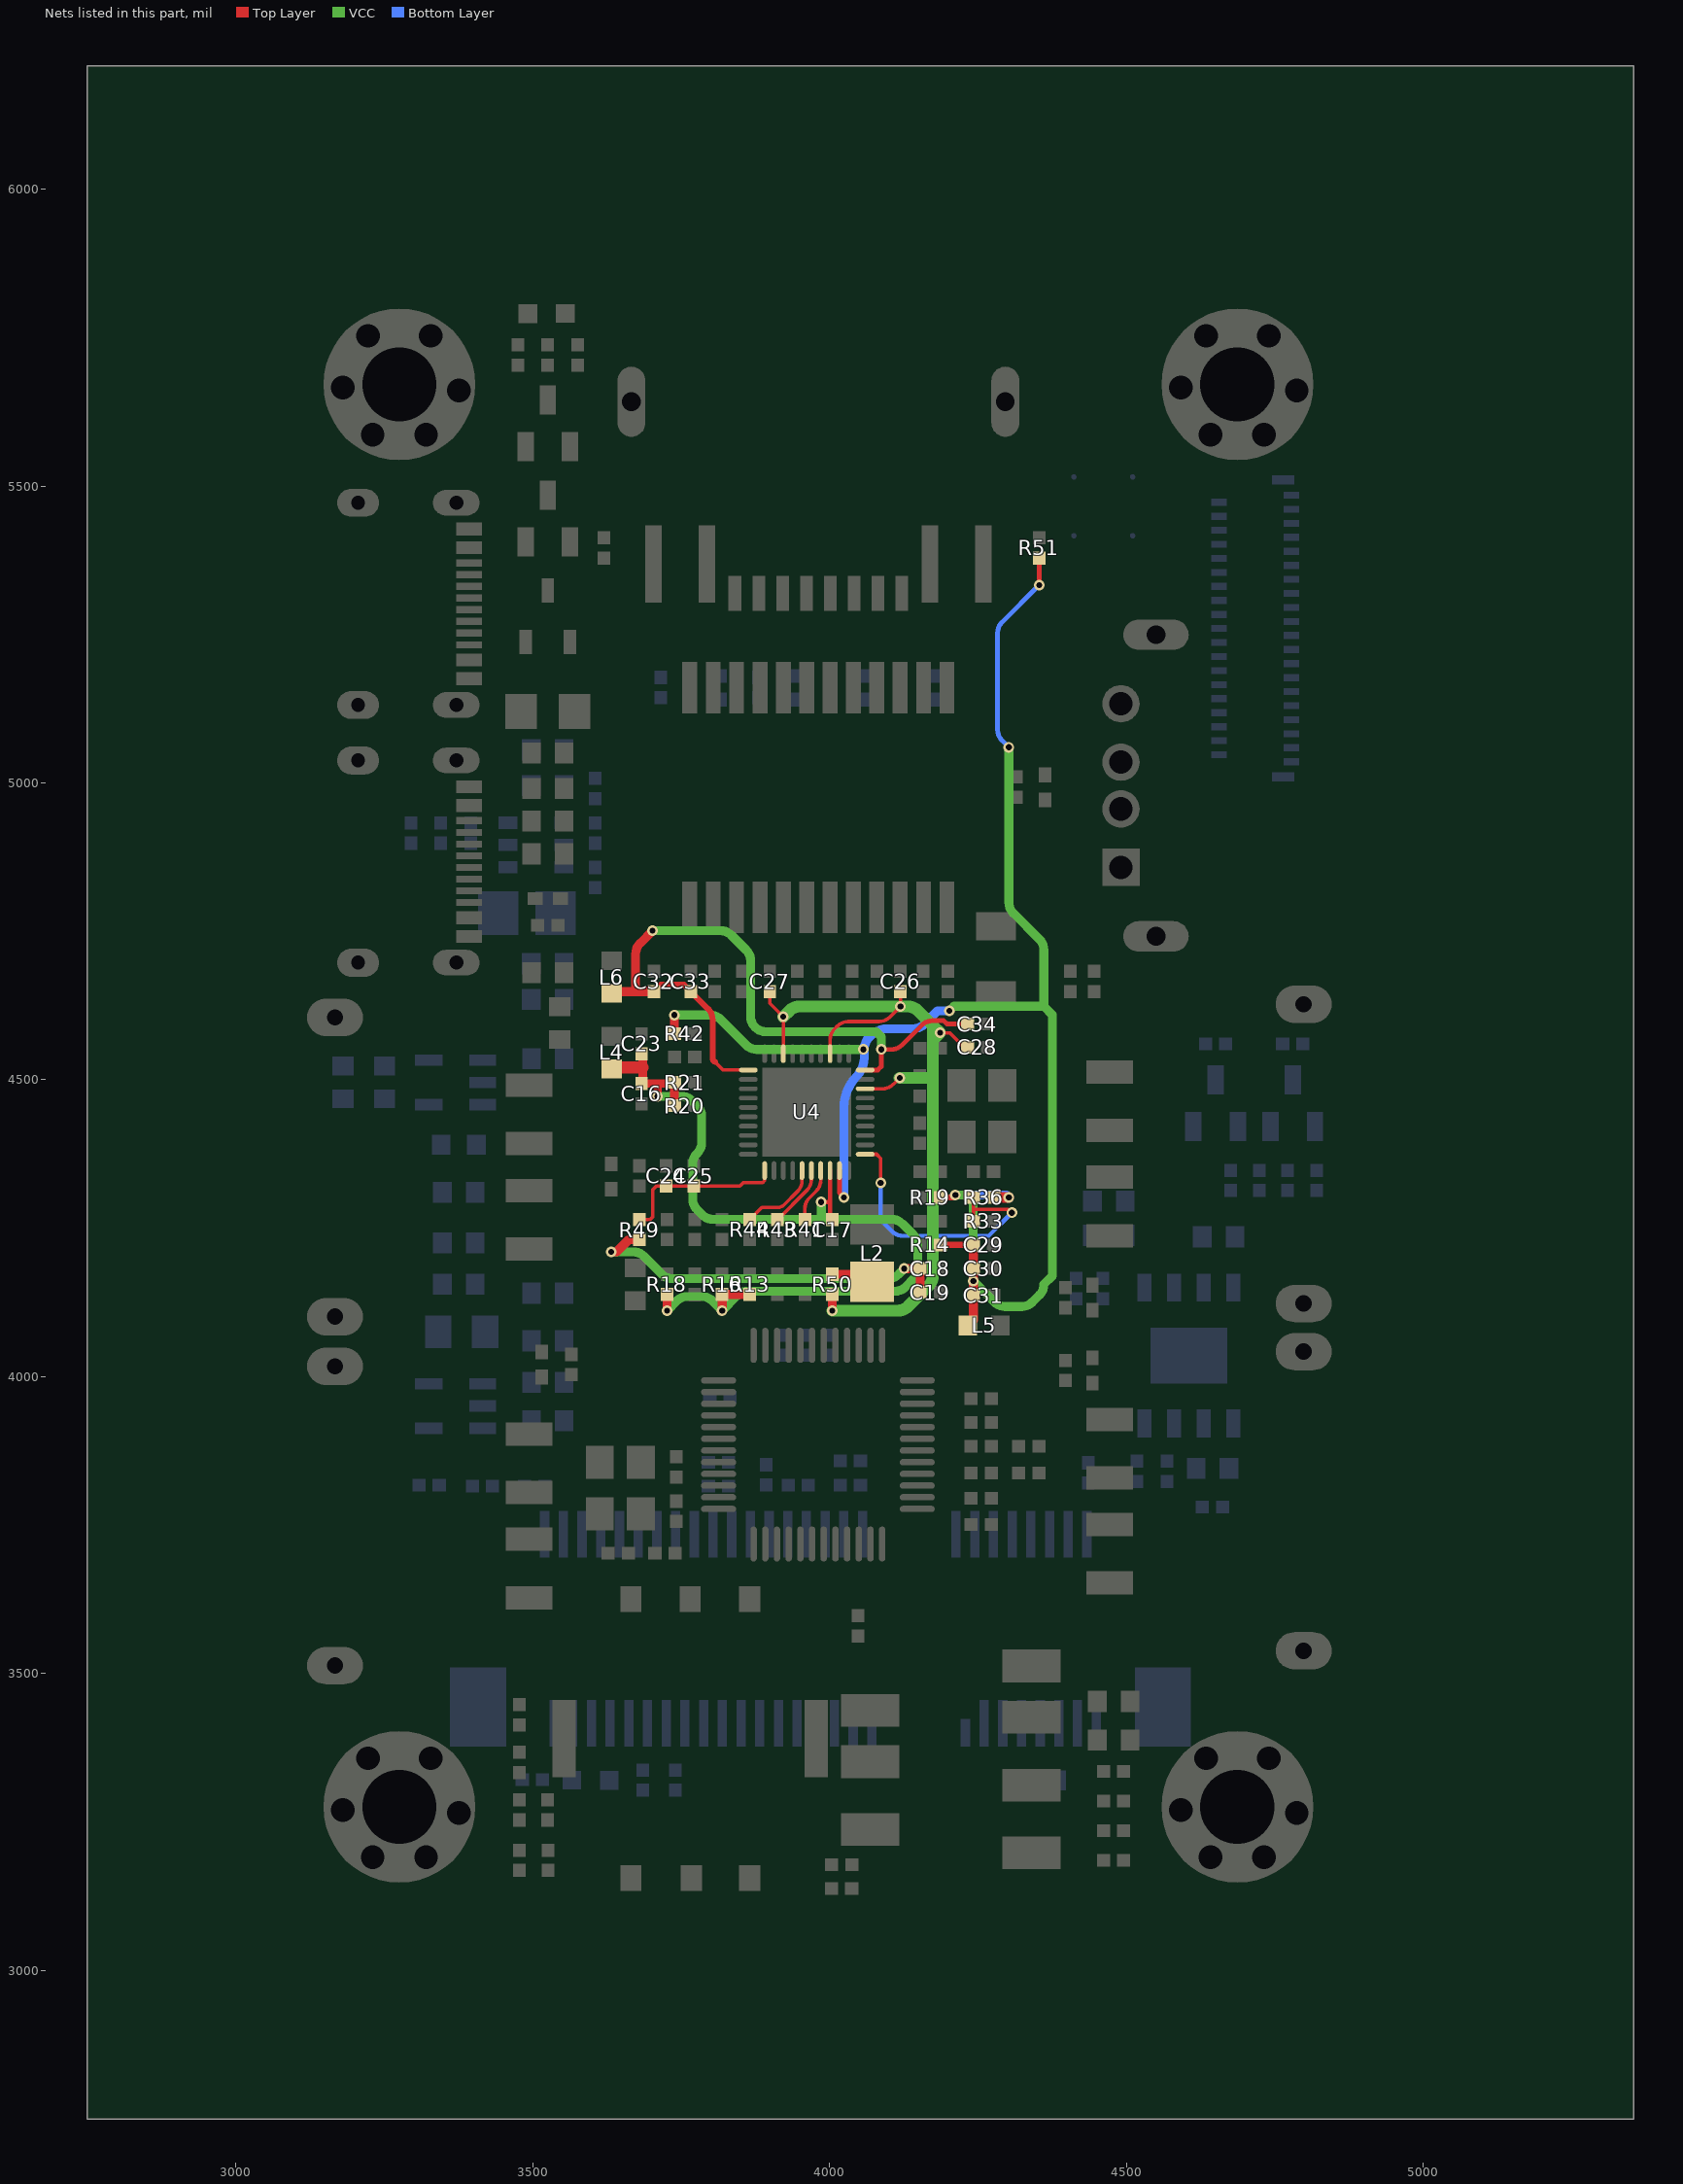
[diagram p0: the nets of this part, all layers, seen from the top]
# Altium PCB MISC84334.PcbDoc (part 3 of 8)
Units mil, origin at the board's own origin, x right, y up, seen from the top; angles counter-clockwise.
Board outline 2605.13 x 3457.4 mil, 4 copper layers (Top Layer, GND, VCC, Bottom Layer), stack 62.447 mil thick; 209 components, 149 nets, 735 pads, 529 vias.

## Footprints (in the part's own frame and the unit in brackets; to place one, negate y for a bottom-side part, rotate by r counter-clockwise, add the part's x,y. Pads: shape width x height; smd on the part's side, far side on the other; paste and mask are expansions set on the pad) (continued)
PCI-SMD_1775862-2 [mm]
  rect 0.4x2 smd: 1(11.8,4.05) 2(11.4,-4.05) 3(11,4.05) 4(10.6,-4.05) 5(10.2,4.05) 6(9.8,-4.05) 7(9.4,4.05) 8(9,-4.05) 9(8.6,4.05) 10(8.2,-4.05) 11(7.8,4.05) 12(7.4,-4.05) 13(7,4.05) 14(6.6,-4.05) 16(5.8,-4.05) 17(2.2,4.05) 18(1.8,-4.05) 19(1.4,4.05) 20(1,-4.05) 21(0.6,4.05) 22(0.2,-4.05) 23(-0.2,4.05) 24(-0.6,-4.05) 25(-1,4.05) 26(-1.4,-4.05) 27(-1.8,4.05) 28(-2.2,-4.05) 29(-2.6,4.05) 30(-3,-4.05) 31(-3.4,4.05) 32(-3.8,-4.05) 33(-4.2,4.05) 34(-4.6,-4.05) 35(-5,4.05) 36(-5.4,-4.05) 37(-5.8,4.05) 38(-6.2,-4.05) 39(-6.6,4.05) 40(-7,-4.05) 41(-7.4,4.05) 42(-7.8,-4.05) 43(-8.2,4.05) 44(-8.6,-4.05) 45(-9,4.05) 46(-9.4,-4.05) 47(-9.8,4.05) 48(-10.2,-4.05) 49(-10.6,4.05) 50(-11,-4.05) 51(-11.4,4.05) 52(-11.8,-4.05)
  rect 0.4x1.2 smd: 15(6.2,4.45)
  rect 2.4x3.4 smd: 53(-14.65,3.35) 53(14.65,3.35)
  Board Outline Layer circle w0.003: c-12.5,0.05 r0.6
  Board Outline Layer circle w0.003: c12.5,0.05 r0.9
  Board Outline Layer region: -11.9,0.05 -11.96,0.31 -12.126,0.519 -12.367,0.635 -12.634,0.635 -12.874,0.519 -13.041,0.31 -13.1,0.05 -13.1,0.05 -13.041,-0.21 -12.874,-0.419 -12.634,-0.535 -12.367,-0.535 -12.126,-0.419 -11.96,-0.21 -11.9,0.05
  Board Outline Layer region: -11.9,0.05 -11.909,0.154 -11.936,0.255 -11.98,0.35 -12.04,0.436 -12.114,0.51 -12.2,0.57 -12.295,0.614 -12.396,0.641 -12.5,0.65 -12.604,0.641 -12.705,0.614 -12.8,0.57 -12.886,0.51 -12.96,0.436 -13.02,0.35 -13.064,0.255 -13.091,0.154 -13.1,0.05 -13.091,-0.054 -13.064,-0.155 -13.02,-0.25 -12.96,-0.336 -12.886,-0.41 -12.8,-0.47 -12.705,-0.514 -12.604,-0.541 -12.5,-0.55 -12.396,-0.541 -12.295,-0.514 -12.2,-0.47 -12.114,-0.41 -12.04,-0.336 -11.98,-0.25 -11.936,-0.155 -11.909,-0.054
  Board Outline Layer region: 13.4,0.05 13.311,0.441 13.061,0.754 12.7,0.927 12.3,0.927 11.939,0.754 11.689,0.441 11.6,0.05 11.6,0.05 11.689,-0.34 11.939,-0.654 12.3,-0.827 12.7,-0.827 13.061,-0.654 13.311,-0.34 13.4,0.05
  Board Outline Layer region: 13.4,0.05 13.39,0.184 13.36,0.315 13.311,0.441 13.244,0.557 13.16,0.662 13.061,0.754 12.95,0.829 12.829,0.888 12.7,0.927 12.567,0.948 12.433,0.948 12.3,0.927 12.171,0.888 12.05,0.829 11.939,0.754 11.84,0.662 11.756,0.557 11.689,0.441 11.64,0.315 11.61,0.184 11.6,0.05 11.61,-0.084 11.64,-0.215 11.689,-0.34 11.756,-0.457 11.84,-0.562 11.939,-0.654 12.05,-0.729 12.171,-0.788 12.3,-0.827 12.433,-0.847 12.567,-0.847 12.7,-0.827 12.829,-0.788 12.95,-0.729 13.061,-0.654 13.16,-0.562 13.244,-0.457 13.311,-0.34 13.36,-0.215 13.39,-0.084
  Multi-Layer board cut-out: -11.9,0.05 -11.96,0.31 -12.126,0.519 -12.367,0.635 -12.634,0.635 -12.874,0.519 -13.041,0.31 -13.1,0.05 -13.1,0.05 -13.041,-0.21 -12.874,-0.419 -12.634,-0.535 -12.367,-0.535 -12.126,-0.419 -11.96,-0.21 -11.9,0.05
  Multi-Layer board cut-out: 13.4,0.05 13.311,0.441 13.061,0.754 12.7,0.927 12.3,0.927 11.939,0.754 11.689,0.441 11.6,0.05 11.6,0.05 11.689,-0.34 11.939,-0.654 12.3,-0.827 12.7,-0.827 13.061,-0.654 13.311,-0.34 13.4,0.05
  silkscreen extent -15,-4.71 15,4.08
R0402 [mm]
  rect 0.566x0.54 smd paste-100 mask+0.051: 1(-0.433,0) 2(0.433,0)
r0402 [mm]
  rect 0.566x0.54 smd paste-100 mask+0.051: 1(-0.433,0) 2(0.433,0)
r0603#1 [mm]
  rect 0.8x0.9 smd: 1(-0.7,0) 2(0.7,0)
r0603#2 [mm]
  rect 0.8x0.9 smd: 1(-0.698,0) 2(0.702,0)
R0603 [mil]
  rect 31.75x34.02 smd paste-3937.01 mask+2: 1(-29.66,0) 2(29.66,0)
R0805 [mm]
  rect 1.133x1.377 smd paste-100 mask+0.051: 1(-1,0) 2(1,0)
r1206 [mil]
  rect 47.54x66.97 smd paste-3937.01 mask+2: 1(-58.22,0) 2(58.22,0)
RJ45-TH_RC01812 [mm]
  rect 0.55x1.5 smd paste-100 mask+0.05: 1(-3.57,-4.1) 2(-2.55,-4.1) 3(-1.53,-4.1) 4(-0.51,-4.1) 5(0.51,-4.1) 6(1.53,-4.1) 7(2.55,-4.1) 8(3.57,-4.1)
  rect 0.7x3.3 smd paste-100 mask+0.05: 9(-7.06,-2.845) 10(-4.77,-2.845) 11(4.77,-2.845) 12(7.06,-2.845)
  oval 1.2x3 hole 0.8 slot 2.2 at 90 deg paste+0 mask+0.05: 13(-8,4.1) 14(8,4.1)
  Board Outline Layer lines w0.254: -8.128,9.271 -6.985,9.271 -6.985,-0.381 6.985,-0.381 6.985,9.271 8.128,9.271
  silkscreen extent -8.1,-3.14 8.13,12.11
SIM-SMD_SMN-304 [mm]
  rect 1x3.29 smd: 1(-5.39,0) 2(5.39,0)
  rect 0.9x1.1 smd: C1(2.54,-5.975) C2(0.051,-5.975) C3(-2.54,-5.975) C5(2.54,5.975) C6(0,5.975) C7(-2.54,5.975)
  Board Outline Layer circle w0.003: c-4.34,-4.155 r0.5
  Board Outline Layer circle w0.003: c4.66,4.145 r0.4
  Board Outline Layer region: -3.84,-4.155 -3.889,-4.372 -4.028,-4.546 -4.229,-4.643 -4.451,-4.643 -4.652,-4.546 -4.79,-4.372 -4.84,-4.155 -4.84,-4.155 -4.79,-3.938 -4.652,-3.764 -4.451,-3.668 -4.229,-3.668 -4.028,-3.764 -3.889,-3.938 -3.84,-4.155
  Board Outline Layer region: -3.84,-4.155 -3.85,-4.253 -3.878,-4.346 -3.924,-4.433 -3.986,-4.509 -4.062,-4.571 -4.149,-4.617 -4.242,-4.645 -4.34,-4.655 -4.438,-4.645 -4.531,-4.617 -4.618,-4.571 -4.694,-4.509 -4.756,-4.433 -4.802,-4.346 -4.83,-4.253 -4.84,-4.155 -4.83,-4.058 -4.802,-3.964 -4.756,-3.877 -4.694,-3.802 -4.618,-3.739 -4.531,-3.693 -4.438,-3.665 -4.34,-3.655 -4.242,-3.665 -4.149,-3.693 -4.062,-3.739 -3.986,-3.802 -3.924,-3.877 -3.878,-3.964 -3.85,-4.058
  Board Outline Layer region: 5.06,4.145 5.02,3.972 4.909,3.832 4.749,3.755 4.571,3.755 4.411,3.832 4.3,3.972 4.26,4.145 4.26,4.145 4.3,4.319 4.411,4.458 4.571,4.535 4.749,4.535 4.909,4.458 5.02,4.319 5.06,4.145
  Board Outline Layer region: 5.06,4.145 5.05,4.056 5.02,3.972 4.973,3.896 4.909,3.832 4.834,3.785 4.749,3.755 4.66,3.745 4.571,3.755 4.486,3.785 4.411,3.832 4.347,3.896 4.3,3.972 4.27,4.056 4.26,4.145 4.27,4.234 4.3,4.319 4.347,4.395 4.411,4.458 4.486,4.506 4.571,4.535 4.66,4.545 4.749,4.535 4.834,4.506 4.909,4.458 4.973,4.395 5.02,4.319 5.05,4.234
  Multi-Layer board cut-out: -3.84,-4.155 -3.889,-4.372 -4.028,-4.546 -4.229,-4.643 -4.451,-4.643 -4.652,-4.546 -4.79,-4.372 -4.84,-4.155 -4.84,-4.155 -4.79,-3.938 -4.652,-3.764 -4.451,-3.668 -4.229,-3.668 -4.028,-3.764 -3.889,-3.938 -3.84,-4.155
  Multi-Layer board cut-out: 5.06,4.145 5.02,3.972 4.909,3.832 4.749,3.755 4.571,3.755 4.411,3.832 4.3,3.972 4.26,4.145 4.26,4.145 4.3,4.319 4.411,4.458 4.571,4.535 4.749,4.535 4.909,4.458 5.02,4.319 5.06,4.145
  silkscreen extent -5.03,-6.15 5.11,6.16
SMD-24_L15.1-W7.1-P1.00-LS10.0-BL [mm]
  rect 0.64x2.2 smd: 1(-5.5,-4.7) 2(-4.5,-4.7) 3(-3.5,-4.7) 4(-2.5,-4.7) 5(-1.5,-4.7) 6(-0.5,-4.7) 7(0.5,-4.7) 8(1.5,-4.7) 9(2.5,-4.7) 10(3.5,-4.7) 11(4.5,-4.7) 12(5.5,-4.7) 13(5.5,4.7) 14(4.5,4.7) 15(3.5,4.7) 16(2.5,4.7) 17(1.5,4.7) 18(0.5,4.7) 19(-0.5,4.7) 20(-1.5,4.7) 21(-2.5,4.7) 22(-3.5,4.7) 23(-4.5,4.7) 24(-5.5,4.7)
  silkscreen extent -7.6,-5 7.6,3.6
SMD_BD4.4-L4.4-D2.8 [mil]
  round 9.02 smd: 1(-49.52,49.5) 1(-49.51,-49.52) 1(49.5,49.52) 1(49.52,-49.5)
  Top Layer region: 3.8,90.43 3.8,60.9 6.05,60.72 8.3,60.45 10.53,60.1 12.75,59.67 14.95,59.15 17.13,58.56 19.29,57.88 21.43,57.13 23.53,56.29 25.6,55.38 27.63,54.39 29.63,53.33 31.59,52.2 33.5,50.99 35.36,49.71 37.18,48.37 38.95,46.96 40.66,45.48 42.32,43.94 43.92,42.34 45.46,40.68 46.94,38.97 48.35,37.2 49.69,35.39 50.97,33.52 52.18,31.61 53.31,29.65 54.37,27.65 55.36,25.62 56.27,23.55 57.11,21.45 57.86,19.31 58.54,17.15 59.13,14.97 59.65,12.77 60.08,10.55 60.43,8.32 60.7,6.07 60.88,3.82 90.41,3.82 90.25,6.56 90.01,9.29 89.69,12.02 89.28,14.73 88.79,17.43 88.22,20.12 87.57,22.79 86.84,25.43 86.02,28.05 85.13,30.65 84.16,33.22 83.12,35.76 81.99,38.26 80.79,40.73 79.52,43.16 78.17,45.56 76.76,47.91 75.27,50.21 73.71,52.47 72.08,54.69 70.39,56.85 68.63,58.96 66.81,61.01 64.93,63.01 62.99,64.95 60.99,66.84 58.94,68.65 56.83,70.41 54.67,72.1 52.45,73.73 50.19,75.29 47.89,76.78 45.54,78.19 43.14,79.54 40.71,80.81 38.24,82.01 35.74,83.14 33.2,84.18 30.63,85.15 28.03,86.04 25.41,86.86 22.77,87.59 20.1,88.24 17.41,88.81 14.71,89.3 12,89.71 9.27,90.03 6.54,90.27
  Top Layer region: -3.8,-90.43 -3.8,-60.9 -6.06,-60.72 -8.3,-60.45 -10.54,-60.1 -12.76,-59.67 -14.96,-59.15 -17.14,-58.56 -19.3,-57.88 -21.43,-57.13 -23.53,-56.29 -25.6,-55.38 -27.64,-54.4 -29.64,-53.33 -31.59,-52.2 -33.51,-50.99 -35.37,-49.71 -37.19,-48.37 -38.96,-46.96 -40.67,-45.48 -42.33,-43.94 -43.93,-42.34 -45.47,-40.68 -46.94,-38.97 -48.35,-37.2 -49.7,-35.39 -50.98,-33.52 -52.18,-31.61 -53.32,-29.65 -54.38,-27.65 -55.37,-25.62 -56.28,-23.55 -57.11,-21.45 -57.87,-19.31 -58.55,-17.15 -59.14,-14.97 -59.66,-12.77 -60.09,-10.55 -60.44,-8.32 -60.7,-6.07 -60.89,-3.82 -90.42,-3.82 -90.26,-6.56 -90.02,-9.29 -89.69,-12.02 -89.28,-14.73 -88.8,-17.43 -88.23,-20.12 -87.57,-22.79 -86.84,-25.43 -86.03,-28.05 -85.14,-30.65 -84.17,-33.22 -83.12,-35.76 -82,-38.26 -80.8,-40.73 -79.53,-43.16 -78.18,-45.56 -76.76,-47.91 -75.27,-50.21 -73.72,-52.47 -72.09,-54.69 -70.4,-56.85 -68.64,-58.96 -66.82,-61.01 -64.94,-63.01 -63,-64.95 -61,-66.84 -58.94,-68.65 -56.83,-70.41 -54.67,-72.1 -52.46,-73.73 -50.2,-75.29 -47.89,-76.78 -45.54,-78.19 -43.15,-79.54 -40.72,-80.81 -38.25,-82.01 -35.74,-83.14 -33.2,-84.18 -30.64,-85.15 -28.04,-86.04 -25.42,-86.86 -22.77,-87.59 -20.1,-88.24 -17.42,-88.81 -14.72,-89.3 -12,-89.71 -9.28,-90.03 -6.54,-90.27
  Top Layer region: -90.43,3.8 -60.9,3.8 -60.72,6.05 -60.45,8.3 -60.1,10.53 -59.67,12.75 -59.15,14.96 -58.56,17.14 -57.88,19.3 -57.13,21.43 -56.29,23.53 -55.38,25.6 -54.4,27.64 -53.33,29.63 -52.2,31.59 -50.99,33.5 -49.72,35.37 -48.37,37.19 -46.96,38.95 -45.48,40.67 -43.94,42.32 -42.34,43.92 -40.69,45.46 -38.97,46.94 -37.2,48.35 -35.39,49.7 -33.52,50.97 -31.61,52.18 -29.65,53.31 -27.65,54.38 -25.62,55.37 -23.55,56.28 -21.45,57.11 -19.31,57.87 -17.15,58.54 -14.98,59.14 -12.77,59.65 -10.55,60.09 -8.32,60.43 -6.07,60.7 -3.82,60.89 -3.82,90.41 -6.56,90.26 -9.29,90.01 -12.02,89.69 -14.73,89.28 -17.43,88.79 -20.12,88.22 -22.79,87.57 -25.43,86.84 -28.06,86.03 -30.65,85.14 -33.22,84.16 -35.76,83.12 -38.26,82 -40.73,80.8 -43.17,79.52 -45.56,78.18 -47.91,76.76 -50.21,75.27 -52.48,73.71 -54.69,72.09 -56.85,70.39 -58.96,68.64 -61.01,66.82 -63.01,64.94 -64.95,62.99 -66.84,60.99 -68.66,58.94 -70.41,56.83 -72.1,54.67 -73.73,52.46 -75.29,50.2 -76.78,47.89 -78.19,45.54 -79.54,43.15 -80.81,40.71 -82.01,38.24 -83.14,35.74 -84.18,33.2 -85.15,30.63 -86.05,28.04 -86.86,25.41 -87.59,22.77 -88.24,20.1 -88.81,17.42 -89.3,14.72 -89.71,12 -90.03,9.27 -90.27,6.54
  Top Layer region: 90.43,-3.8 60.9,-3.8 60.72,-6.05 60.45,-8.3 60.1,-10.53 59.67,-12.75 59.15,-14.96 58.56,-17.14 57.88,-19.3 57.13,-21.43 56.29,-23.53 55.38,-25.6 54.4,-27.64 53.33,-29.63 52.2,-31.59 50.99,-33.5 49.71,-35.37 48.37,-37.19 46.96,-38.95 45.48,-40.67 43.94,-42.32 42.34,-43.92 40.68,-45.46 38.97,-46.94 37.2,-48.35 35.38,-49.69 33.52,-50.97 31.61,-52.18 29.65,-53.32 27.65,-54.38 25.62,-55.36 23.55,-56.28 21.45,-57.11 19.31,-57.87 17.15,-58.54 14.97,-59.14 12.77,-59.65 10.55,-60.08 8.32,-60.44 6.07,-60.7 3.82,-60.88 3.82,-90.41 6.56,-90.26 9.29,-90.01 12.02,-89.69 14.73,-89.28 17.43,-88.79 20.12,-88.22 22.78,-87.57 25.43,-86.84 28.05,-86.03 30.65,-85.14 33.22,-84.16 35.76,-83.12 38.26,-81.99 40.73,-80.8 43.16,-79.52 45.56,-78.18 47.91,-76.76 50.21,-75.27 52.47,-73.71 54.69,-72.09 56.85,-70.39 58.96,-68.64 61.01,-66.82 63.01,-64.94 64.95,-62.99 66.83,-60.99 68.65,-58.94 70.41,-56.83 72.1,-54.67 73.73,-52.46 75.29,-50.2 76.78,-47.89 78.19,-45.54 79.54,-43.15 80.81,-40.71 82.01,-38.24 83.14,-35.74 84.18,-33.2 85.15,-30.63 86.04,-28.04 86.85,-25.41 87.59,-22.77 88.24,-20.1 88.81,-17.42 89.3,-14.71 89.7,-12 90.03,-9.27 90.27,-6.54
  Board Outline Layer circle w0.1: c0,0 r59.05
  Board Outline Layer region: -59.06,0 -53.21,-25.62 -36.82,-46.17 -13.14,-57.57 13.14,-57.57 36.82,-46.17 53.2,-25.62 59.05,0 59.05,0 53.2,25.62 36.82,46.17 13.14,57.57 -13.14,57.57 -36.82,46.17 -53.21,25.62 -59.06,0
  Board Outline Layer region: -59.06,0 -58.66,-6.86 -57.47,-13.62 -55.5,-20.2 -52.78,-26.5 -49.34,-32.45 -45.24,-37.96 -40.53,-42.96 -35.27,-47.37 -29.53,-51.14 -23.39,-54.23 -16.94,-56.57 -10.26,-58.16 -3.44,-58.96 3.43,-58.96 10.25,-58.16 16.94,-56.57 23.39,-54.23 29.53,-51.14 35.26,-47.37 40.52,-42.96 45.24,-37.96 49.34,-32.45 52.77,-26.5 55.49,-20.2 57.46,-13.62 58.65,-6.86 59.05,0 58.65,6.86 57.46,13.62 55.49,20.2 52.77,26.5 49.34,32.45 45.24,37.96 40.52,42.96 35.26,47.37 29.53,51.14 23.39,54.23 16.94,56.57 10.25,58.16 3.43,58.96 -3.44,58.96 -10.26,58.16 -16.94,56.57 -23.39,54.23 -29.53,51.14 -35.27,47.37 -40.53,42.96 -45.24,37.96 -49.34,32.45 -52.78,26.5 -55.5,20.2 -57.47,13.62 -58.66,6.86
  Multi-Layer board cut-out: -59.06,0 -53.21,-25.62 -36.82,-46.17 -13.14,-57.57 13.14,-57.57 36.82,-46.17 53.2,-25.62 59.05,0 59.05,0 53.2,25.62 36.82,46.17 13.14,57.57 -13.14,57.57 -36.82,46.17 -53.21,25.62 -59.06,0
  silkscreen extent -100,-100 100,100
SOT-23-3_L2.9-W1.3-P1.90-LS2.4-BR [mm]
  rect 1.25x0.7 smd: 1(1,-0.95) 2(1,0.95) 3(-1,0)
SOT-23-3_L3.0-W1.7-P0.95-LS2.9-BR [mil]
  rect 40.85x20.95 smd: 1(43.36,-37.4) 2(43.36,37.4) 3(-43.36,0)
SOT-23-5_L3.0-W1.7-P0.95-LS2.8-BL [mm]
  rect 0.49x1.157 smd: 1(-0.95,-1.154) 2(0,-1.154) 3(0.95,-1.154)
  rect 0.49x1.175 smd: 4(0.95,1.154) 5(-0.95,1.154)
  silkscreen extent -1.8,-1.29 1.53,0.85
TSOT-23-6_L2.9-W1.6-P0.95-LS2.8-BR [mm]
  rect 0.8x0.532 smd: 1(1.2,-0.95) 2(1.2,0) 3(1.2,0.95) 4(-1.2,0.95) 5(-1.2,0) 6(-1.2,-0.95)
  silkscreen extent 1.14,-1.82 1.44,-1.52
USB-A-SMD_AF-SMT-SHORT [mm]
  rect 1x2 smd paste-100 mask+0.051: 1(-3.5,4.15) 2(-1,4.15) 3(1,4.15) 4(3.5,4.15)
  oval 1.6x2.4 hole 0.7 slot 1.6 at 90 deg copper offset 0.001,0: SH1(6.399,-4.15)
  oval 1.6x2.4 hole 0.7 slot 1.6 at 90 deg copper offset -0.001,0: SH2(-6.399,-4.15)
  silkscreen extent -7.29,-6.37 7.3,4.43
USB-A-TH_AF-10.0-HC6.3 [mm]
  rect 1.6x1.6 hole 1 paste+0 mask+0.05: 1(-3.5,0.75)
  round 1.6 hole 1 paste+0 mask+0.05: 2(-1,0.75) 3(1,0.75) 4(3.5,0.75)
  oval 1.3x2.8 hole 0.8 slot 2.1 at 90 deg paste+0 mask+0.05: 5(-6.45,-0.75) 6(6.45,-0.75)
  silkscreen extent -6.6,-9.27 6.6,1.02
USB-C-SMD_TYPE-C-6PIN-2MD-073 [mm]
  rect 0.55x1.1 smd paste-100 mask+0.05: 1(-3.2,2.375) 2(-2.4,2.375) 11(2.4,2.375) 12(3.2,2.375)
  rect 0.3x1.1 smd paste-100 mask+0.05: 3(-1.75,2.375) 4(-1.25,2.375) 5(-0.75,2.375) 6(-0.25,2.375) 7(0.25,2.375) 8(0.75,2.375) 9(1.25,2.375) 10(1.75,2.375)
  oval 1.2x1.8 hole 0.6 slot 1.2 at 90 deg paste+0 mask+0.05: 13(-4.325,-2.375) 14(4.325,-2.375)
  oval 1.1x2 hole 0.6 slot 1.5 at 90 deg paste+0 mask+0.05: 13(-4.325,1.825) 14(4.325,1.825)
  Board Outline Layer circle w0.003: c-2.89,1.305 r0.35
  Board Outline Layer circle w0.003: c2.89,1.305 r0.35
  Board Outline Layer region: -2.89,1.655 -2.738,1.62 -2.616,1.523 -2.549,1.383 -2.549,1.227 -2.616,1.087 -2.738,0.99 -2.89,0.955 -2.89,0.955 -3.042,0.99 -3.164,1.087 -3.231,1.227 -3.231,1.383 -3.164,1.523 -3.042,1.62 -2.89,1.655
  Board Outline Layer region: -2.89,1.655 -2.812,1.646 -2.738,1.62 -2.672,1.579 -2.616,1.523 -2.575,1.457 -2.549,1.383 -2.54,1.305 -2.549,1.227 -2.575,1.153 -2.616,1.087 -2.672,1.031 -2.738,0.99 -2.812,0.964 -2.89,0.955 -2.968,0.964 -3.042,0.99 -3.108,1.031 -3.164,1.087 -3.205,1.153 -3.231,1.227 -3.24,1.305 -3.231,1.383 -3.205,1.457 -3.164,1.523 -3.108,1.579 -3.042,1.62 -2.968,1.646
  Board Outline Layer region: 2.89,1.655 3.042,1.62 3.164,1.523 3.231,1.383 3.231,1.227 3.164,1.087 3.042,0.99 2.89,0.955 2.89,0.955 2.738,0.99 2.616,1.087 2.549,1.227 2.549,1.383 2.616,1.523 2.738,1.62 2.89,1.655
  Board Outline Layer region: 2.89,1.655 2.968,1.646 3.042,1.62 3.108,1.579 3.164,1.523 3.205,1.457 3.231,1.383 3.24,1.305 3.231,1.227 3.205,1.153 3.164,1.087 3.108,1.031 3.042,0.99 2.968,0.964 2.89,0.955 2.812,0.964 2.738,0.99 2.672,1.031 2.616,1.087 2.575,1.153 2.549,1.227 2.54,1.305 2.549,1.383 2.575,1.457 2.616,1.523 2.672,1.579 2.738,1.62 2.812,1.646
  Multi-Layer board cut-out: -2.89,1.655 -2.738,1.62 -2.616,1.523 -2.549,1.383 -2.549,1.227 -2.616,1.087 -2.738,0.99 -2.89,0.955 -2.89,0.955 -3.042,0.99 -3.164,1.087 -3.231,1.227 -3.231,1.383 -3.164,1.523 -3.042,1.62 -2.89,1.655
  Multi-Layer board cut-out: 2.89,1.655 3.042,1.62 3.164,1.523 3.231,1.383 3.231,1.227 3.164,1.087 3.042,0.99 2.89,0.955 2.89,0.955 2.738,0.99 2.616,1.087 2.549,1.227 2.549,1.383 2.616,1.523 2.738,1.62 2.89,1.655
  silkscreen extent -4.5,-4.97 4.57,0.6
WQFN-40_L5.0-W5.0-P0.4-BL-EP [mm]
  oval 0.2x0.8 smd paste-100 mask+0.051: 1(-1.801,-2.499) 2(-1.4,-2.499) 3(-1.001,-2.499) 4(-0.599,-2.499) 5(-0.201,-2.499) 6(0.201,-2.499) 7(0.599,-2.499) 8(1.001,-2.499) 9(1.4,-2.499) 10(1.801,-2.499) 21(1.801,2.499) 22(1.4,2.499) 23(1.001,2.499) 24(0.599,2.499) 25(0.201,2.499) 26(-0.201,2.499) 27(-0.599,2.499) 28(-1.001,2.499) 29(-1.4,2.499) 30(-1.801,2.499)
  oval 0.8x0.2 smd paste-100 mask+0.051: 11(2.499,-1.801) 12(2.499,-1.4) 13(2.499,-1.001) 14(2.499,-0.599) 15(2.499,-0.201) 16(2.499,0.201) 17(2.499,0.599) 18(2.499,1.001) 19(2.499,1.4) 20(2.499,1.801) 31(-2.499,1.801) 32(-2.499,1.4) 33(-2.499,1.001) 34(-2.499,0.599) 35(-2.499,0.201) 36(-2.499,-0.201) 37(-2.499,-0.599) 38(-2.499,-1.001) 39(-2.499,-1.4) 40(-2.499,-1.801)
  rect 3.8x3.8 smd paste-100 mask+0.051: 41(0,0)
  silkscreen extent -2.7,-3.35 2.7,2.7

## Via types
v1: diameter 18, hole 10, Top Layer to Bottom Layer, 529 vias

## Nets (pads, with @x,y where several pads share a name; then routed paths per layer and width w, separated by ;. In a path a pad name is that pad's centre, name@x,y a point inside that pad or via, vN(x,y) a via of type N, cw(c..) or ccw(c..) an arc to the next point about the centre after c; other vN are vias at no path point)
1V05_AVDD_PHY: C26.2 C27.2 C28.2 R50.2 U4.3 U4.8 U4.38 | length 1435.7
  Top Layer w6: C27.2@3899.65,4648.55 3899.65,4628.83 3915.04,4613.44 cw(c3897.36,4595.77) 3920.46,4605.33 cw(c3897.36,4595.77) 3922.36,4595.77 U4.8@3922.36,4543.99 ; U4.3@4001.16,4543.99 4001.16,4567.7 cw(c4026.16,4567.7) 4008.48,4585.38 4013.97,4590.87 cw(c4031.65,4573.19) 4031.65,4598.19 4083.94,4598.19 ccw(c4083.94,4623.19) 4101.61,4605.51 v1(4119.79,4623.69) C26.2@4119.79,4648.55 ; U4.38@4060.16,4484.99 4089.74,4484.99 ccw(c4089.74,4509.99) 4107.41,4492.31 v1(4118.29,4503.19) ; v1(4186.29,4579.19) 4202.34,4579.19 C28.2@4232.44,4549.09
  Top Layer w15: v1(4005.09,4111.19) R50.2@4005.09,4138.55
  VCC w20: v1(3922.36,4606.12) 3932.61,4616.37 cw(c3950.28,4598.69) 3950.28,4623.69 v1(4119.79,4623.69) 4131.44,4623.69 cw(c4131.44,4598.69) 4149.11,4616.37 4174.29,4591.19 ; v1(4005.09,4111.19) 4114.94,4111.19 ccw(c4114.94,4136.19) 4132.61,4118.51 4166.97,4152.87 ccw(c4149.29,4170.55) 4174.29,4170.55 4174.29,4502.71 ; v1(4118.29,4503.19) 4173.81,4503.19 4174.29,4502.71 ; 4174.29,4502.71 4174.29,4567.19 ; 4174.29,4567.19 v1(4186.29,4579.19) 4174.29,4591.19 ; 4174.29,4567.19 4174.29,4591.19
1V05_DVDD_PHY: C24.2 C25.2 R49.1 U4.21 | length 281.6
  Top Layer w6: R49.1@3680.09,4264.89 3698.03,4264.89 3702.29,4269.15 3702.29,4314.96 3708.38,4321.05 C24.2@3725.09,4321.05 C25.2@3771.52,4321.05 3849.15,4321.05 3855.15,4327.05 3887.64,4327.05 3890.86,4330.27 U4.21@3890.86,4347.19
1V05_PHY: C18.2 C19.2 L2.2 R49.2 R50.1 | length 711.4
  Top Layer w15: v1(3632.29,4210.19) 3641.34,4210.19 3661.96,4230.81 R49.2@3680.09,4230.81 ; R50.1@4005.09,4172.63 4059.06,4172.63 L2.2@4071.95,4159.74 ; v1(4126.27,4182.09) C18.2@4152.55,4182.09 cw(c4152.55,4181.85) 4152.79,4181.85 C19.2@4152.79,4142.09
  VCC w15: v1(3632.29,4210.19) 3669.94,4210.19 cw(c3669.94,4185.19) 3687.61,4202.87 3717.97,4172.51 ccw(c3735.65,4190.19) 3735.65,4165.19 4099.01,4165.19 ccw(c4099.01,4190.19) 4116.69,4172.51 v1(4126.27,4182.09)
1V8_DVDD_PHY: C16.2 C17.2 C23.2 L4.1 R13.1 R16.1 R18.1 R20.1 R21.1 U4.28 | length 1614.2
  Top Layer w8: v1(3986.29,4294.19) 3999.89,4294.19 4001.16,4292.92 ; U4.28@4001.16,4347.19 4001.16,4292.92 ; C17.2@4005.09,4264.89 4001.16,4268.82 4001.16,4292.92
  Top Layer w14: C16.2@3685.59,4493.75 3710.31,4493.75 ; v1(3710.31,4472.19) 3710.31,4493.75 ; R21.1@3737.21,4493.75 3710.31,4493.75
  Top Layer w15: L4.1@3633.09,4518.3 L4.1@3635.75,4520.96 ; C16.2@3685.59,4493.75 3685.59,4520.96 C23.2@3685.59,4543.55 ; v1(3726.52,4111.19) R18.1@3726.52,4138.55 ; R21.1@3737.21,4493.75 R21.1@3739.05,4495.59 R20.1@3739.05,4456.33 ; v1(3819.38,4111.19) R16.1@3819.38,4138.55 R13.1@3865.8,4138.55
  Top Layer w20: L4.1@3635.75,4520.96 3685.59,4520.96
  VCC w15: v1(3710.31,4472.19) 3750.94,4472.19 cw(c3750.94,4447.19) 3768.61,4464.87 3777.47,4456.01 cw(c3759.79,4438.34) 3784.79,4438.34 3784.79,4394.05 cw(c3759.79,4394.05) 3777.47,4376.37 3777.11,4376.01 ccw(c3794.79,4358.34) 3769.79,4358.34 3769.79,4299.05 ccw(c3794.79,4299.05) 3777.11,4281.37 3785.97,4272.51 ccw(c3803.65,4290.19) 3803.65,4265.19 3986.29,4265.19 ; v1(3726.52,4111.19) 3743.2,4127.87 cw(c3760.87,4110.19) 3760.87,4135.19 3785.02,4135.19 cw(c3785.02,4110.19) 3802.7,4127.87 v1(3819.38,4111.19) 3845.05,4136.87 cw(c3862.73,4119.19) 3862.73,4144.19 4110.94,4144.19 ccw(c4110.94,4169.19) 4128.61,4151.51 4141.45,4164.35 ccw(c4123.77,4182.02) 4148.77,4182.02 4148.77,4221.36 ccw(c4123.77,4221.36) 4141.45,4239.04 4122.61,4257.87 ccw(c4104.94,4240.19) 4104.94,4265.19 3986.29,4265.19 ; v1(3986.29,4294.19) 3986.29,4265.19
3V3_AVDD_PHY: C32.2 C33.2 C34.2 L6.1 U4.11 U4.40 | length 1220.9
  Top Layer w6: 3807.29,4530.19 3820.99,4516.49 U4.11@3863.36,4516.49
  Top Layer w8: U4.40@4060.16,4516.49 4081.57,4516.49 4087.29,4522.21 v1(4087.29,4551.19) 4104.39,4551.19 ccw(c4104.39,4576.19) 4122.07,4558.51 4155.85,4592.3 cw(c4173.53,4574.62) 4173.53,4599.62 4192.55,4599.62 4198.08,4594.09 C34.2@4232.44,4594.09
  Top Layer w10: C32.2@3704.09,4648.55 3715.73,4660.19 3754.91,4660.19 C33.2@3766.55,4648.55 3795.97,4619.13 cw(c3778.29,4601.45) 3803.29,4601.45 3803.29,4534.19 3807.29,4530.19
  Top Layer w15: L6.1@3633.09,4645.54 3636.11,4648.55 3673.6,4648.55 ; v1(3702.29,4751.19) 3680.92,4729.82 ccw(c3698.6,4712.14) 3673.6,4712.14 3673.6,4648.55 ; C32.2@3704.09,4648.55 3673.6,4648.55
  VCC w15: v1(3702.29,4751.19) 3816.94,4751.19 cw(c3816.94,4726.19) 3834.61,4743.87 3859.97,4718.51 cw(c3842.29,4700.84) 3867.29,4700.84 3867.29,4606.55 ccw(c3892.29,4606.55) 3874.61,4588.87 3874.97,4588.51 ccw(c3892.65,4606.19) 3892.65,4581.19 4078.5,4581.19 4087.29,4572.4 v1(4087.29,4551.19)
3V3_DVDD_PHY: C29.2 C30.2 C31.2 L5.1 R14.2 R19.2 R36.2 R42.2 R51.1 U4.29 | length 2967.6
  Top Layer w8: U4.29@4016.86,4347.19 4016.86,4309.62 v1(4024.29,4302.19) ; R51.1@4353.17,5378.55 4353.29,5378.43 v1(4353.29,5333.19)
  Top Layer w10: R14.2@4186.75,4222.09 C29.2@4242.55,4222.09 ; R19.2@4186.81,4302.09 4208.29,4302.09 v1(4212.29,4306.09)
  Top Layer w15: R42.2@3739.05,4578.09 v1(3739.05,4609.19) ; L5.1@4233.01,4086.09 4242.55,4095.63 C31.2@4242.55,4137.09 v1(4242.55,4161.07) C30.2@4242.55,4182.09 C29.2@4242.55,4222.09
  Top Layer w18: R36.2@4276.63,4302.09 v1(4302.29,4302.09)
  VCC w15: v1(3739.05,4609.19) 3798.94,4609.19 cw(c3798.94,4584.19) 3816.61,4601.87 3859.97,4558.51 ccw(c3877.65,4576.19) 3877.65,4551.19 v1(4057.29,4551.19) ; v1(4202.29,4616.19) 4209.95,4623.85 4361.29,4623.85 ; v1(4212.29,4306.09) 4228.79,4306.09 4242.29,4292.59 4242.29,4161.33 v1(4242.55,4161.07) 4278.11,4125.51 ccw(c4295.79,4143.19) 4295.79,4118.19 4323.94,4118.19 ccw(c4323.94,4143.19) 4341.61,4125.51 4353.97,4137.87 ccw(c4336.29,4155.55) 4361.29,4155.55 4375.59,4169.85 4375.59,4609.55 4361.29,4623.85 ; v1(4302.29,5060.19) 4302.29,4798.61 ccw(c4327.29,4798.61) 4309.61,4780.93 4353.97,4736.57 cw(c4336.29,4718.9) 4361.29,4718.9 4361.29,4623.85
  Bottom Layer w8: v1(4302.29,5060.19) 4290.61,5071.87 cw(c4308.29,5089.55) 4283.29,5089.55 4283.29,5252.84 cw(c4308.29,5252.84) 4290.61,5270.51 v1(4353.29,5333.19)
  Bottom Layer w15: v1(4024.29,4302.19) 4024.29,4452.47 cw(c4101.19,4452.47) 4045.59,4505.59 ccw(c4010.82,4538.81) v1(4057.29,4551.19) cw(c4098.56,4544.36) 4098.56,4586.19 4141.94,4586.19 ccw(c4141.94,4611.19) 4159.61,4593.51 4182.29,4616.19 v1(4202.29,4616.19) ; v1(4212.29,4306.09) 4298.29,4306.09 v1(4302.29,4302.09)
$2N2719: R33.1 R36.1 U4.31 | length 486.3
  Top Layer w6: U4.31@4060.16,4374.69 4079.5,4374.69 4086.29,4367.9 v1(4086.29,4326.19) ; R33.1@4242.55,4262.09 4242.55,4280.88 ; R36.1@4242.55,4302.09 4242.55,4280.88 ; v1(4307.29,4276.19) 4301.66,4281.83 4243.5,4281.83 4242.55,4280.88
  Bottom Layer w7: v1(4086.29,4326.19) 4086.29,4274.55 ccw(c4111.29,4274.55) 4093.61,4256.87 4105.97,4244.51 ccw(c4123.65,4262.19) 4123.65,4237.19 4268.29,4237.19 v1(4307.29,4276.19)
$2N2795: R41.1 U4.27 | length 91.2
  Top Layer w6: R41.1@3958.66,4264.89 3958.66,4283.21 cw(c3983.66,4283.21) 3965.98,4300.88 3978.04,4312.94 ccw(c3960.36,4330.62) 3985.36,4330.62 U4.27@3985.36,4347.19
$2N2796: R43.1 U4.26 | length 105.5
  Top Layer w6: R43.1@3912.23,4264.89 3912.99,4264.89 3962.34,4314.24 ccw(c3944.66,4331.92) 3969.66,4331.92 U4.26@3969.66,4347.19
$2N2797: R44.1 U4.25 | length 136.5
  Top Layer w6: R44.1@3865.8,4264.89 3865.99,4264.89 3886.29,4285.19 3913.4,4285.19 ccw(c3913.4,4299.07) 3923.21,4289.26 3946.54,4312.58 ccw(c3928.86,4330.26) 3953.86,4330.26 U4.25@3953.86,4347.19